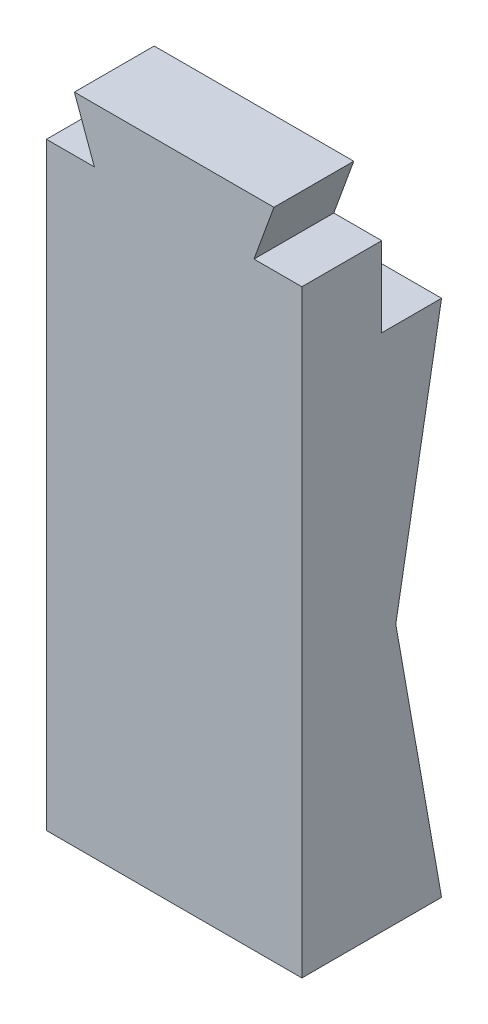
from build123d import *

# Parameters (mm, degrees)
BOSS_EXTRUDE1_DEPTH = 20
BOSS_EXTRUDE2_DEPTH = 64


with BuildPart() as part:
    # Sketch1 → Boss-Extrude1 (new body)
    with BuildSketch(Plane.XY):
        Polygon((-27.262159038, -0.780894157), (-27.262159038, -150.780894157), (36.737840962, -150.780894157), (36.737840962, -0.780894157), (24.737840962, -0.780894157), (29.737840962, 12.95649294), (-20.262159038, 12.95649294), (-15.262159038, -0.780894157), align=None)
    extrude(amount=BOSS_EXTRUDE1_DEPTH)

    # Sketch2 → Boss-Extrude2 (add)
    with BuildSketch(Plane(origin=(36.737840962, 0, 0), x_dir=(0, 0, -1), z_dir=(1, 0, 0))):
        Polygon((0, -150.780894157), (15, -150.780894157), (3.538746274, -85.783666039), (15, -20.780894157), (0, -20.780894157), align=None)
    extrude(amount=-BOSS_EXTRUDE2_DEPTH)


solid = part.part
